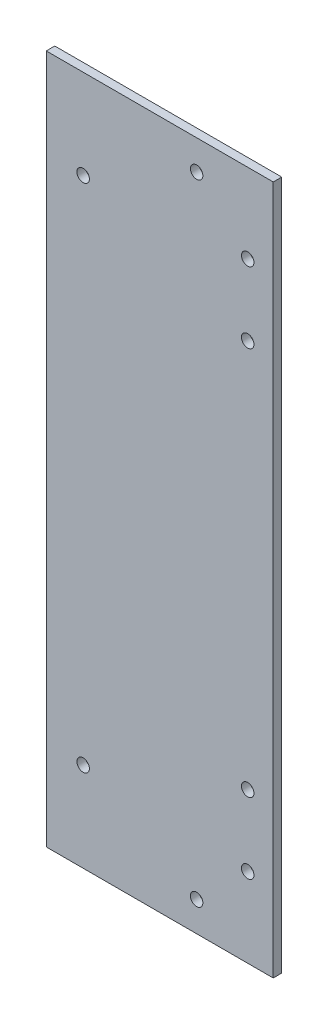
SolidWorks part; units mm, degrees
ref_plane "前视基准面" through (0, 0, 0) normal (0, 0, 1) x (1, 0, 0)
ref_plane "上视基准面" through (0, 0, 0) normal (0, 1, 0) x (1, 0, 0)
ref_plane "右视基准面" through (0, 0, 0) normal (1, 0, 0) x (0, 0, -1)
sketch "草图1" plane through (0, 0, 0) normal (0, 0, 1) x (1, 0, 0)
  line L1 (40, -121.5) -> (-40, -121.5)
  line L2 (40, -121.5) -> (40, 121.5)
  line L3 (40, 121.5) -> (-40, 121.5)
  line L4 (-40, -121.5) -> (-40, 121.5)
  line L5 (40, -121.5) -> (-40, 121.5) construction
  line L6 (40, 121.5) -> (-40, -121.5) construction
  point P0 (0, 0)
  dimension "D1" = 80
  dimension "D2" = 243
extrude "凸台-拉伸1" add sketch "草图1" along normal blind 3
sketch "草图4" plane through (0, 0, 0) normal (0, 0, -1) x (-1, 0, 0)
  line L0 (-31, -121.5) -> (-31, -93.5) construction
  line L1 (40, -121.5) -> (-40, -121.5) construction
  line L2 (-31, -93.5) -> (-31, -68.5) construction
  line L3 (-40, -121.5) -> (-40, 121.5) construction
  circle A0 centre (-31, -68.5) radius 2.2
  circle A1 centre (-31, -93.5) radius 2.2
  dimension "D1" = 4.4
  dimension "D2" = 25
  dimension "D3" = 28
  dimension "D4" = 9
extrude "切除-拉伸2" cut sketch "草图4" against normal blind 10
mirror "镜向1" about plane through (0, 0, 0) normal (0, 1, 0) of "切除-拉伸2"
sketch "草图5" plane through (0, 0, 0) normal (0, 0, -1) x (-1, 0, 0)
  line L0 (-13, 111) -> (27, 111) construction
  line L1 (27, 111) -> (27, -111) construction
  line L2 (27, -111) -> (-13, -111) construction
  line L3 (40, 121.5) -> (40, -121.5) construction
  line L4 (0, 0) -> (27, 0) construction
  line L5 (0, 0) -> (27, 0) construction
  circle A0 centre (-13, 111) radius 2.2
  circle A1 centre (-13, -111) radius 2.2
  circle A2 centre (27, 90) radius 2.2
  circle A3 centre (27, -90) radius 2.2
  dimension "D4" = 4.4
  dimension "D5" = 180
  dimension "D1" = 40
  dimension "D2" = 13
  dimension "D3" = 222
  dimension "D6" = 90
extrude "切除-拉伸3" cut sketch "草图5" against normal blind 10
